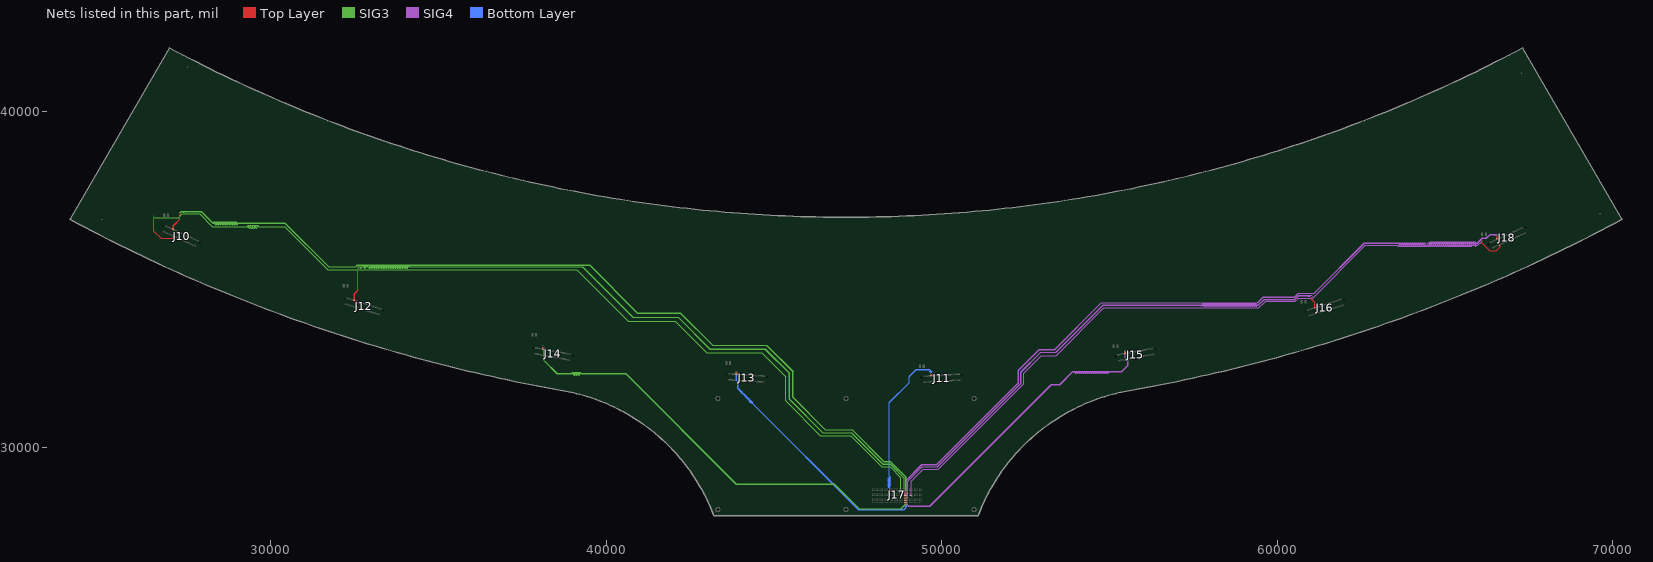
[diagram p0: the nets of this part, all layers, seen from the top]
# Altium PCB MISC86329.PcbDoc (part 4 of 11)
Units mil, origin at the board's own origin, x right, y up, seen from the top; angles counter-clockwise.
Board outline 46247.15 x 13937.21 mil, 6 copper layers (Top Layer, GND2, SIG3, SIG4, POWER5, Bottom Layer); 17 components, 210 nets, 908 pads, 1109 vias.

## Via types
v1: diameter 24, hole 12, Top Layer to Bottom Layer, 684 vias
v2: diameter 18, hole 9, Top Layer to Bottom Layer, 425 vias

## Nets (pads, with @x,y where several pads share a name; then routed paths per layer and width w, separated by ;. In a path a pad name is that pad's centre, name@x,y a point inside that pad or via, vN(x,y) a via of type N, cw(c..) or ccw(c..) an arc to the next point about the centre after c; other vN are vias at no path point) (continued)
DATAIN1P_CH7: J17.E7 J18.15 | length 23896.2
  Top Layer w5: J17.E7@49087.89,28568.8 v2(49111.69,28545) ; 66093,36150.5 66093,36104 66333,35864 66527,35864 66644,35981 66644,36016.48 J18.15@66618.61,36041.87
  SIG4 w5: v2(49111.69,28545) 49091.69,28565 49091.69,28998 49444.69,29351 49892.14,29351 52448,31906.86 52448,32213.86 52969.14,32735 53408.14,32735 54832.14,34159 59452.14,34159 59651.14,34358 60542.14,34358 60640.14,34456 61055.14,34456 62623.14,36024 63571.86,36024 63594.86,36001 63616.14,36001 63631.5,36016.36 63631.5,36049.43 63636.07,36054 63646.93,36054 63651.5,36049.43 63651.5,36004.43 63661.93,35994 63681.07,35994 63691.5,36004.43 63691.5,36049.43 63696.07,36054 63706.93,36054 63711.5,36049.43 63711.5,36004.43 63721.93,35994 63741.07,35994 63751.5,36004.43 63751.5,36049.43 63756.07,36054 63766.93,36054 63771.5,36049.43 63771.5,36004.43 63781.93,35994 63801.07,35994 63811.5,36004.43 63811.5,36049.43 63816.07,36054 63826.93,36054 63831.5,36049.43 63831.5,36004.43 63841.93,35994 63861.07,35994 63871.5,36004.43 63871.5,36049.43 63876.07,36054 63886.93,36054 63891.5,36049.43 63891.5,36004.43 63901.93,35994 63921.07,35994 63931.5,36004.43 63931.5,36049.43 63936.07,36054 63946.93,36054 63951.5,36049.43 63951.5,36004.43 63961.93,35994 63981.07,35994 63991.5,36004.43 63991.5,36049.43 63996.07,36054 64006.93,36054 64011.5,36049.43 64011.5,36004.43 64021.93,35994 64041.07,35994 64051.5,36004.43 64051.5,36049.43 64056.07,36054 64066.93,36054 64071.5,36049.43 64071.5,36004.43 64081.93,35994 64101.07,35994 64111.5,36004.43 64111.5,36049.43 64116.07,36054 64126.93,36054 64131.5,36049.43 64131.5,36004.43 64141.93,35994 64161.07,35994 64171.5,36004.43 64171.5,36049.43 64176.07,36054 64186.93,36054 64191.5,36049.43 64191.5,36004.43 64201.93,35994 64221.07,35994 64231.5,36004.43 64231.5,36049.43 64236.07,36054 64246.93,36054 64251.5,36049.43 64251.5,36004.43 64261.93,35994 64281.07,35994 64291.5,36004.43 64291.5,36049.43 64296.07,36054 64306.93,36054 64311.5,36049.43 64311.5,36004.43 64321.93,35994 64341.07,35994 64351.5,36004.43 64351.5,36049.43 64356.07,36054 64366.93,36054 64371.5,36049.43 64371.5,36004.43 64381.93,35994 64401.07,35994 64411.5,36004.43 64411.5,36019.43 64416.07,36024 64426.93,36024 64431.5,36019.43 64431.5,36004.43 64441.93,35994 64461.07,35994 64471.5,36004.43 64471.5,36019.43 64476.07,36024 64486.93,36024 64491.5,36019.43 64491.5,36004.43 64501.93,35994 64521.07,35994 64531.5,36004.43 64531.5,36049.43 64536.07,36054 64546.93,36054 64551.5,36049.43 64551.5,36004.43 64561.93,35994 64581.07,35994 64591.5,36004.43 64591.5,36019.43 64596.07,36024 64606.93,36024 64611.5,36019.43 64611.5,36004.43 64621.93,35994 64641.07,35994 64651.5,36004.43 64651.5,36019.43 64656.07,36024 64666.93,36024 64671.5,36019.43 64671.5,36004.43 64681.93,35994 64701.07,35994 64711.5,36004.43 64711.5,36019.43 64716.07,36024 64726.93,36024 64731.5,36019.43 64731.5,36004.43 64741.93,35994 64761.07,35994 64771.5,36004.43 64771.5,36019.43 64776.07,36024 64786.93,36024 64791.5,36019.43 64791.5,36004.43 64801.93,35994 64821.07,35994 64831.5,36004.43 64831.5,36019.43 64836.07,36024 64846.93,36024 64851.5,36019.43 64851.5,36004.43 64861.93,35994 64881.07,35994 64891.5,36004.43 64891.5,36019.43 64896.07,36024 64906.93,36024 64911.5,36019.43 64911.5,36004.43 64921.93,35994 64941.07,35994 64951.5,36004.43 64951.5,36019.43 64956.07,36024 64966.93,36024 64971.5,36019.43 64971.5,36004.43 64981.93,35994 65001.07,35994 65011.5,36004.43 65011.5,36019.43 65016.07,36024 65026.93,36024 65031.5,36019.43 65031.5,36004.43 65041.93,35994 65061.07,35994 65071.5,36004.43 65071.5,36019.43 65076.07,36024 65086.93,36024 65091.5,36019.43 65091.5,36004.43 65101.93,35994 65121.07,35994 65131.5,36004.43 65131.5,36019.43 65136.07,36024 65146.93,36024 65151.5,36019.43 65151.5,36004.43 65161.93,35994 65181.07,35994 65191.5,36004.43 65191.5,36019.43 65196.07,36024 65206.93,36024 65211.5,36019.43 65211.5,36004.43 65221.93,35994 65241.07,35994 65251.5,36004.43 65251.5,36019.43 65256.07,36024 65266.93,36024 65271.5,36019.43 65271.5,36004.43 65281.93,35994 65301.07,35994 65311.5,36004.43 65311.5,36019.43 65316.07,36024 65326.93,36024 65331.5,36019.43 65331.5,36004.43 65341.93,35994 65361.07,35994 65371.5,36004.43 65371.5,36019.43 65376.07,36024 65386.93,36024 65391.5,36019.43 65391.5,36004.43 65401.93,35994 65421.07,35994 65431.5,36004.43 65431.5,36019.43 65436.07,36024 65446.93,36024 65451.5,36019.43 65451.5,36004.43 65461.93,35994 65481.07,35994 65491.5,36004.43 65491.5,36019.43 65496.07,36024 65506.93,36024 65511.5,36019.43 65511.5,36004.43 65521.93,35994 65541.07,35994 65551.5,36004.43 65551.5,36019.43 65556.07,36024 65566.93,36024 65571.5,36019.43 65571.5,36004.43 65581.93,35994 65601.07,35994 65611.5,36004.43 65611.5,36019.43 65616.07,36024 65626.93,36024 65631.5,36019.43 65631.5,36004.43 65641.93,35994 65661.07,35994 65671.5,36004.43 65671.5,36019.43 65676.07,36024 65686.93,36024 65691.5,36019.43 65691.5,36004.43 65701.93,35994 65721.07,35994 65731.5,36004.43 65731.5,36019.43 65736.07,36024 65746.93,36024 65751.5,36019.43 65751.5,36004.43 65761.93,35994 65781.07,35994 65791.5,36004.43 65791.5,36019.43 65796.07,36024 65893,36024 65898,36019 65898,36007.06 65903,36002.06 65913,36002.06 65918,36007.06 65918,36019 65923,36024 65980,36024 66093,36137 66093,36143 ; 66093,36146 66093,36143 ; v2@66100,36157 66093,36150 66093,36143
  other v2: 66099.5,36157
DATAIN2N_CH0: J10.18 J17.G11 | length 27866.7
  Top Layer w5: J10.18@27107.16,36497.31 27107.16,36524.91 27120,36537.75 27120,36615 27304,36799 27304,36956.5 v2(27310.5,36963) ; J17.G11@48887.89,28668.8 v2(48911.69,28692.61)
  SIG3 w5: v2(27310.5,36963) 27304,36969.5 27304,36986 27347,37029 27388,37029 27403,37029 27408,37024 27408,37014.52 27413,37009.52 27423,37009.52 27428,37014.52 27428,37024 27433,37029 27935.86,37029 28280.86,36684 28313.82,36684 28325.5,36695.68 28325.5,36718.18 28331.32,36724 28344.68,36724 28350.5,36718.18 28350.5,36655.68 28362.18,36644 28383.82,36644 28395.5,36655.68 28395.5,36718.18 28401.32,36724 28414.68,36724 28420.5,36718.18 28420.5,36655.68 28432.18,36644 28453.82,36644 28465.5,36655.68 28465.5,36718.18 28471.32,36724 28484.68,36724 28490.5,36718.18 28490.5,36655.68 28502.18,36644 28523.82,36644 28535.5,36655.68 28535.5,36718.18 28541.32,36724 28554.68,36724 28560.5,36718.18 28560.5,36655.68 28572.18,36644 28593.82,36644 28605.5,36655.68 28605.5,36718.18 28611.32,36724 28624.68,36724 28630.5,36718.18 28630.5,36655.68 28642.18,36644 28663.82,36644 28675.5,36655.68 28675.5,36718.18 28681.32,36724 28694.68,36724 28700.5,36718.18 28700.5,36655.68 28712.18,36644 28733.82,36644 28745.5,36655.68 28745.5,36718.18 28751.32,36724 28764.68,36724 28770.5,36718.18 28770.5,36655.68 28782.18,36644 28803.82,36644 28815.5,36655.68 28815.5,36718.18 28821.32,36724 28834.68,36724 28840.5,36718.18 28840.5,36655.68 28852.18,36644 28873.82,36644 28885.5,36655.68 28885.5,36718.18 28891.32,36724 28904.68,36724 28910.5,36718.18 28910.5,36655.68 28922.18,36644 28943.82,36644 28955.5,36655.68 28955.5,36718.18 28961.32,36724 28974.68,36724 28980.5,36718.18 28980.5,36655.68 28992.18,36644 29013.82,36644 29025.5,36655.68 29025.5,36678.18 29031.32,36684 30428.86,36684 31731.86,35381 32545.14,35381 32596.14,35432 39506.86,35432 40930.86,34008 42208.86,34008 43173.86,33043 44780,33043 45560,32263 45560,31492.86 46528.86,30524 47328.86,30524 48274.86,29578 48465,29578 48931.69,29111.31 48931.69,28712.61 v2(48911.69,28692.61)
DATAIN2N_CH1: J12.18 J17.F11 | length 23094.8
  Top Layer w5: J12.18@32516.49,34376.54 32516.49,34403 32511,34408.49 32511,34584 32607,34680 32607,35344.5 v2(32613.5,35351) ; J17.F11@48887.89,28618.8 v2(48911.69,28642.61)
  SIG3 w5: v2(32613.5,35351) 32607,35357.5 32607,35366.86 32622.14,35382 32643,35382 32655.5,35382 32674.25,35382 32680.5,35375.75 32680.5,35349.42 32686.75,35343.17 32699.25,35343.17 32705.5,35349.42 32705.5,35375.75 32711.75,35382 32760.82,35382 32772.5,35393.68 32772.5,35406.18 32778.32,35412 32791.68,35412 32797.5,35406.18 32797.5,35354.13 32809.18,35342.46 32830.82,35342.46 32842.5,35354.13 32842.5,35406.18 32848.32,35412 32861.68,35412 32867.5,35406.18 32867.5,35393.68 32879.18,35382 32913,35382 32927.18,35382 32933,35376.18 32933,35354.13 32944.68,35342.46 32966.32,35342.46 32978,35354.13 32978,35406.18 32983.82,35412 32997.18,35412 33003,35406.18 33003,35354.13 33014.68,35342.46 33036.32,35342.46 33048,35354.13 33048,35406.18 33053.82,35412 33067.18,35412 33073,35406.18 33073,35354.13 33084.68,35342.46 33106.32,35342.46 33118,35354.13 33118,35406.18 33123.82,35412 33137.18,35412 33143,35406.18 33143,35354.13 33154.68,35342.46 33176.32,35342.46 33188,35354.13 33188,35406.18 33193.82,35412 33207.18,35412 33213,35406.18 33213,35354.13 33224.68,35342.46 33246.32,35342.46 33258,35354.13 33258,35406.18 33263.82,35412 33277.18,35412 33283,35406.18 33283,35354.13 33294.68,35342.46 33316.32,35342.46 33328,35354.13 33328,35406.18 33333.82,35412 33347.18,35412 33353,35406.18 33353,35354.13 33364.68,35342.46 33386.32,35342.46 33398,35354.13 33398,35406.18 33403.82,35412 33417.18,35412 33423,35406.18 33423,35354.13 33434.68,35342.46 33456.32,35342.46 33468,35354.13 33468,35406.18 33473.82,35412 33487.18,35412 33493,35406.18 33493,35354.13 33504.68,35342.46 33526.32,35342.46 33538,35354.13 33538,35406.18 33543.82,35412 33557.18,35412 33563,35406.18 33563,35354.13 33574.68,35342.46 33596.32,35342.46 33608,35354.13 33608,35406.18 33613.82,35412 33627.18,35412 33633,35406.18 33633,35354.13 33644.68,35342.46 33666.32,35342.46 33678,35354.13 33678,35406.18 33683.82,35412 33697.18,35412 33703,35406.18 33703,35354.13 33714.68,35342.46 33736.32,35342.46 33748,35354.13 33748,35406.18 33753.82,35412 33767.18,35412 33773,35406.18 33773,35354.13 33784.68,35342.46 33806.32,35342.46 33818,35354.13 33818,35406.18 33823.82,35412 33837.18,35412 33843,35406.18 33843,35354.13 33854.68,35342.46 33876.32,35342.46 33888,35354.13 33888,35406.18 33893.82,35412 33907.18,35412 33913,35406.18 33913,35354.13 33924.68,35342.46 33946.32,35342.46 33958,35354.13 33958,35406.18 33963.82,35412 33977.18,35412 33983,35406.18 33983,35354.13 33994.68,35342.46 34016.32,35342.46 34028,35354.13 34028,35406.18 34033.82,35412 34047.18,35412 34053,35406.18 34053,35354.13 34064.68,35342.46 34086.32,35342.46 34098,35354.13 34098,35406.18 34103.82,35412 34117.18,35412 34123,35406.18 34123,35393.68 34134.68,35382 39295.86,35382 40801.86,33876 42143.86,33876 43088.86,32931 44733,32931 45456,32208 45456,31434.86 46452.86,30438 47310.86,30438 48246.86,29502 48464,29502 48881,29085 48881,28676 48904.96,28652.04 48911.69,28645.31 v2(48911.69,28642.61)
DATAIN2N_CH2: J14.18 J17.B11 | length 13802
  Top Layer w5: v2(38142.5,33020) 38136,33013.5 38136,32958 38143.96,32950.04 J14.18@38143.96,32930.8 ; J17.B11@48887.89,28418.8 v2(48911.69,28395)
  SIG3 w5: v2@38142,33018 38136,33012 38136,32962.14 38146,32952.14 38146,32926.75 38152.25,32920.5 38157.54,32920.5 38163.79,32914.25 38163.79,32901.75 38157.54,32895.5 38152.25,32895.5 38146,32889.25 38146,32606 38541,32211 38988.68,32211 38994.5,32216.82 38994.5,32239.32 39006.18,32251 39027.82,32251 39039.5,32239.32 39039.5,32176.82 39045.32,32171 39058.68,32171 39064.5,32176.82 39064.5,32239.32 39076.18,32251 39097.82,32251 39109.5,32239.32 39109.5,32176.82 39115.32,32171 39128.68,32171 39134.5,32176.82 39134.5,32239.32 39146.18,32251 39167.82,32251 39179.5,32239.32 39179.5,32176.82 39185.32,32171 39198.68,32171 39204.5,32176.82 39204.5,32239.32 39216.18,32251 39237.82,32251 39249.5,32239.32 39249.5,32216.82 39255.32,32211 40584,32211 43873,28922 46805,28922 47547,28180 48783.69,28180 48931.69,28328 48931.69,28375 v2(48911.69,28395)
DATAIN2N_CH3: J13.18 J17.A11 | length 7737.2
  Top Layer w5: v2(43901.45,32250) 43894.95,32243.5 43894.95,32220.72 43905.67,32210 J13.18@43905.67,32181.66 ; J17.A11@48887.89,28368.8 v2(48911.69,28345)
  Bottom Layer w5: v2@43901,32247 43895,32241 43895,32204.75 43901.25,32198.5 43907.59,32198.5 43913.84,32192.25 43913.84,32179.75 43907.59,32173.5 43901.25,32173.5 43895,32167.25 43895,32001 43931,31965 43931,31754 43943.45,31741.55 43948.15,31741.55 43953.45,31746.85 43966.44,31746.85 43978.2,31735.08 43978.2,31722.1 43972.9,31716.8 43972.9,31712.1 43978.81,31706.19 43983.51,31706.19 43988.81,31711.49 44001.79,31711.49 44013.56,31699.73 44013.56,31686.74 44008.26,31681.44 44008.26,31676.74 44014.17,31670.83 44018.86,31670.83 44024.17,31676.14 44037.15,31676.14 44048.91,31664.37 44048.91,31651.39 44043.61,31646.09 44043.61,31641.39 44049.52,31635.48 44054.22,31635.48 44059.52,31640.78 44072.5,31640.78 44084.27,31629.01 44084.27,31616.03 44078.97,31610.73 44078.97,31606.03 44084.88,31600.12 44089.57,31600.12 44094.88,31605.43 44107.86,31605.43 44119.62,31593.66 44119.62,31580.68 44114.32,31575.38 44114.32,31570.68 44120.23,31564.77 44124.93,31564.77 44130.23,31570.07 44143.21,31570.07 44154.98,31558.3 44154.98,31545.32 44149.68,31540.02 44149.68,31535.32 44155.59,31529.41 44160.28,31529.41 44165.59,31534.72 44178.57,31534.72 44190.34,31522.95 44190.34,31509.97 44185.03,31504.66 44185.03,31499.97 44190.94,31494.06 44195.64,31494.06 44200.94,31499.36 44213.92,31499.36 44225.69,31487.59 44225.69,31474.61 44220.39,31469.31 44220.39,31464.61 44226.3,31458.7 44230.99,31458.7 44236.3,31464.01 44249.28,31464.01 44261.05,31452.24 44261.05,31439.26 44255.74,31433.95 44255.74,31429.26 44261.65,31423.35 44266.35,31423.35 44271.65,31428.65 44284.63,31428.65 44296.4,31416.88 44296.4,31403.9 44276.96,31384.46 44276.96,31379.76 44282.87,31373.85 44287.56,31373.85 44307.01,31393.29 44319.99,31393.29 44331.76,31381.53 44331.76,31368.55 44312.31,31349.1 44312.31,31344.4 44318.22,31338.49 44322.92,31338.49 44342.36,31357.94 44355.34,31357.94 44367.11,31346.17 44367.11,31333.19 44361.81,31327.89 44361.81,31323.19 47525,28160 48880,28160 48931.69,28211.69 48931.69,28228.18 48928.37,28231.5 48920.87,28231.5 48911.69,28240.68 48911.69,28257.32 48920.87,28266.5 48948.37,28266.5 48951.69,28269.82 48951.69,28278.18 48948.37,28281.5 48940.87,28281.5 48931.69,28290.68 48931.69,28325 v2(48911.69,28345)
DATAIN2N_CH4: J11.18 J17.H20 | length 5091.6
  Top Layer w5: v2(48414.09,28742.61) J17.H20@48437.89,28718.8 ; 49705.01,32196.5 49705.01,32175.72 49715.73,32165 J11.18@49715.73,32140.28
  Bottom Layer w5: v2(48414.09,28742.61) 48434.09,28762.61 48434.09,28813.93 48431.02,28817 48413.02,28817 48404.09,28825.93 48404.09,28848.07 48413.02,28857 48461.02,28857 48464.09,28860.07 48464.09,28873.93 48461.02,28877 48413.02,28877 48404.09,28885.93 48404.09,28908.07 48413.02,28917 48461.02,28917 48464.09,28920.07 48464.09,28933.93 48461.02,28937 48413.02,28937 48404.09,28945.93 48404.09,28968.07 48413.02,28977 48461.02,28977 48464.09,28980.07 48464.09,28993.93 48461.02,28997 48413.02,28997 48404.09,29005.93 48404.09,29028.07 48413.02,29037 48461.02,29037 48464.09,29040.07 48464.09,29053.93 48461.02,29057 48413.02,29057 48404.09,29065.93 48404.09,29088.07 48413.02,29097 48461.02,29097 48464.09,29100.07 48464.09,29113.93 48461.02,29117 48434.09,29143.91 48434.09,31343.09 49028,31937 49028,32120 49239,32331 49631.14,32331 49705,32257.14 49705,32210 v2@49713,32202
  other v2: 49711.51,32203
DATAIN2N_CH5: J15.18 J17.C11 | length 10126
  Top Layer w5: J17.C11@48887.89,28468.8 v2(48911.69,28445) ; 55474,32875.5 55474,32846.53 55487.53,32833 J15.18@55487.53,32807.27
  SIG4 w5: v2(48911.69,28445) 48933,28423.69 48933,28324.86 49000.86,28257 49653.14,28257 53274.14,31878 53526.14,31878 53908.14,32260 53967.43,32260 53972,32255.43 53972,32231.38 53982.43,32220.95 54001.57,32220.95 54012,32231.38 54012,32255.43 54016.57,32260 54027.43,32260 54032,32255.43 54032,32231.38 54042.43,32220.95 54061.57,32220.95 54072,32231.38 54072,32255.43 54076.57,32260 54087.43,32260 54092,32255.43 54092,32231.38 54102.43,32220.95 54121.57,32220.95 54132,32231.38 54132,32255.43 54136.57,32260 54147.43,32260 54152,32255.43 54152,32231.38 54162.43,32220.95 54181.57,32220.95 54192,32231.38 54192,32255.43 54196.57,32260 54207.43,32260 54212,32255.43 54212,32231.38 54222.43,32220.95 54241.57,32220.95 54252,32231.38 54252,32255.43 54256.57,32260 54267.43,32260 54272,32255.43 54272,32231.38 54282.43,32220.95 54301.57,32220.95 54312,32231.38 54312,32255.43 54316.57,32260 54327.43,32260 54332,32255.43 54332,32231.38 54342.43,32220.95 54361.57,32220.95 54372,32231.38 54372,32255.43 54376.57,32260 54387.43,32260 54392,32255.43 54392,32231.38 54402.43,32220.95 54421.57,32220.95 54432,32231.38 54432,32255.43 54436.57,32260 54447.43,32260 54452,32255.43 54452,32231.38 54462.43,32220.95 54481.57,32220.95 54492,32231.38 54492,32255.43 54496.57,32260 54507.43,32260 54512,32255.43 54512,32231.38 54522.43,32220.95 54541.57,32220.95 54552,32231.38 54552,32255.43 54556.57,32260 54567.43,32260 54572,32255.43 54572,32231.38 54582.43,32220.95 54601.57,32220.95 54612,32231.38 54612,32255.43 54616.57,32260 54627.43,32260 54632,32255.43 54632,32231.38 54642.43,32220.95 54661.57,32220.95 54672,32231.38 54672,32255.43 54676.57,32260 54687.43,32260 54692,32255.43 54692,32231.38 54702.43,32220.95 54721.57,32220.95 54732,32231.38 54732,32255.43 54736.57,32260 54747.43,32260 54752,32255.43 54752,32231.38 54762.43,32220.95 54781.57,32220.95 54792,32231.38 54792,32255.43 54796.57,32260 54807.43,32260 54812,32255.43 54812,32231.38 54822.43,32220.95 54841.57,32220.95 54852,32231.38 54852,32255.43 54856.57,32260 54867.43,32260 54872,32255.43 54872,32231.38 54882.43,32220.95 54901.57,32220.95 54912,32231.38 54912,32255.43 54916.57,32260 54927.43,32260 54932,32255.43 54932,32231.38 54942.43,32220.95 54961.57,32220.95 54972,32231.38 54972,32255.43 54976.57,32260 55371,32260 55561,32450 55561,32580.14 55474,32667.14 55474,32765 55474,32795 55474,32825 55474,32840 55474,32850 55474,32876 v2@55478,32880
  other v2: 55480.5,32882
DATAIN2N_CH6: J16.18 J17.D11 | length 18294.2
  Top Layer w5: J17.D11@48887.89,28518.8 v2(48911.69,28495) ; 61030,34491.5 61030,34416 61119,34327 61119,34188.72 J16.18@61135.02,34172.7
  SIG4 w5: v2(48911.69,28495) 48938.36,28495 48954.86,28511.5 48964.05,28511.5 48982,28529.45 48982,28994.14 49420.86,29433 49872,29433 52362,31923 52362,32254 52952,32844 53404,32844 54809,34249 57710,34249 57730,34229 57750.86,34229 57763,34241.14 57763,34268.57 57773.43,34279 57792.57,34279 57803,34268.57 57803,34223.57 57807.57,34219 57818.43,34219 57823,34223.57 57823,34268.57 57833.43,34279 57852.57,34279 57863,34268.57 57863,34223.57 57867.57,34219 57878.43,34219 57883,34223.57 57883,34268.57 57893.43,34279 57912.57,34279 57923,34268.57 57923,34223.57 57927.57,34219 57938.43,34219 57943,34223.57 57943,34268.57 57953.43,34279 57972.57,34279 57983,34268.57 57983,34223.57 57987.57,34219 57998.43,34219 58003,34223.57 58003,34268.57 58013.43,34279 58032.57,34279 58043,34268.57 58043,34223.57 58047.57,34219 58058.43,34219 58063,34223.57 58063,34268.57 58073.43,34279 58092.57,34279 58103,34268.57 58103,34223.57 58107.57,34219 58118.43,34219 58123,34223.57 58123,34268.57 58133.43,34279 58152.57,34279 58163,34268.57 58163,34223.57 58167.57,34219 58178.43,34219 58183,34223.57 58183,34268.57 58193.43,34279 58212.57,34279 58223,34268.57 58223,34223.57 58227.57,34219 58238.43,34219 58243,34223.57 58243,34268.57 58253.43,34279 58272.57,34279 58283,34268.57 58283,34223.57 58287.57,34219 58298.43,34219 58303,34223.57 58303,34268.57 58313.43,34279 58332.57,34279 58343,34268.57 58343,34223.57 58347.57,34219 58358.43,34219 58363,34223.57 58363,34268.57 58373.43,34279 58392.57,34279 58403,34268.57 58403,34223.57 58407.57,34219 58418.43,34219 58423,34223.57 58423,34268.57 58433.43,34279 58452.57,34279 58463,34268.57 58463,34223.57 58467.57,34219 58478.43,34219 58483,34223.57 58483,34268.57 58493.43,34279 58512.57,34279 58523,34268.57 58523,34223.57 58527.57,34219 58538.43,34219 58543,34223.57 58543,34268.57 58553.43,34279 58572.57,34279 58583,34268.57 58583,34223.57 58587.57,34219 58598.43,34219 58603,34223.57 58603,34268.57 58613.43,34279 58632.57,34279 58643,34268.57 58643,34223.57 58647.57,34219 58658.43,34219 58663,34223.57 58663,34268.57 58673.43,34279 58692.57,34279 58703,34268.57 58703,34223.57 58707.57,34219 58718.43,34219 58723,34223.57 58723,34268.57 58733.43,34279 58752.57,34279 58763,34268.57 58763,34223.57 58767.57,34219 58778.43,34219 58783,34223.57 58783,34268.57 58793.43,34279 58812.57,34279 58823,34268.57 58823,34223.57 58827.57,34219 58838.43,34219 58843,34223.57 58843,34268.57 58853.43,34279 58872.57,34279 58883,34268.57 58883,34223.57 58887.57,34219 58898.43,34219 58903,34223.57 58903,34268.57 58913.43,34279 58932.57,34279 58943,34268.57 58943,34223.57 58947.57,34219 58958.43,34219 58963,34223.57 58963,34268.57 58973.43,34279 58992.57,34279 59003,34268.57 59003,34223.57 59007.57,34219 59018.43,34219 59023,34223.57 59023,34268.57 59033.43,34279 59052.57,34279 59063,34268.57 59063,34223.57 59067.57,34219 59078.43,34219 59083,34223.57 59083,34268.57 59093.43,34279 59112.57,34279 59123,34268.57 59123,34223.57 59127.57,34219 59138.43,34219 59143,34223.57 59143,34268.57 59153.43,34279 59172.57,34279 59183,34268.57 59183,34223.57 59187.57,34219 59198.43,34219 59203,34223.57 59203,34268.57 59213.43,34279 59232.57,34279 59243,34268.57 59243,34223.57 59247.57,34219 59258.43,34219 59263,34223.57 59263,34268.57 59273.43,34279 59292.57,34279 59303,34268.57 59303,34223.57 59307.57,34219 59318.43,34219 59323,34223.57 59323,34268.57 59333.43,34279 59352.57,34279 59363,34268.57 59363,34223.57 59367.57,34219 59378.43,34219 59383,34223.57 59383,34238.57 59393.43,34249 59434.86,34249 59605.86,34420 60522,34420 60638,34536 61017.14,34536 61030,34523.14 61030,34509 61036,34503 v2@61036,34500
  other v2: 61036.5,34498
DATAIN2N_CH7: J17.E11 J18.18 | length 23893.9
  Top Layer w5: J17.E11@48887.89,28568.8 v2(48911.69,28545) ; 66555.34,36303.5 66555.34,36261.68 66564,36253.01 66564,36226.22 J18.18@66574.01,36216.2
  SIG4 w5: v2(48911.69,28545) 48931.69,28565 48931.69,29018.83 49412.86,29500 49854,29500 52286,31932 52286,32309.14 52905.86,32929 53366,32929 54755,34318 59409,34318 59581,34490 60516,34490 60631,34605 61104,34605 62597,36098 64392,36098 64411,36079 64477.86,36079 64496.86,36098 64538.43,36098 64543,36102.57 64543,36117.57 64553.43,36128 64572.57,36128 64583,36117.57 64583,36072.57 64587.57,36068 64598.43,36068 64603,36072.57 64603,36117.57 64613.43,36128 64632.57,36128 64643,36117.57 64643,36072.57 64647.57,36068 64658.43,36068 64663,36072.57 64663,36117.57 64673.43,36128 64692.57,36128 64703,36117.57 64703,36072.57 64707.57,36068 64718.43,36068 64723,36072.57 64723,36117.57 64733.43,36128 64752.57,36128 64763,36117.57 64763,36072.57 64767.57,36068 64778.43,36068 64783,36072.57 64783,36117.57 64793.43,36128 64812.57,36128 64823,36117.57 64823,36072.57 64827.57,36068 64838.43,36068 64843,36072.57 64843,36117.57 64853.43,36128 64872.57,36128 64883,36117.57 64883,36072.57 64887.57,36068 64898.43,36068 64903,36072.57 64903,36117.57 64913.43,36128 64932.57,36128 64943,36117.57 64943,36072.57 64947.57,36068 64958.43,36068 64963,36072.57 64963,36117.57 64973.43,36128 64992.57,36128 65003,36117.57 65003,36072.57 65007.57,36068 65018.43,36068 65023,36072.57 65023,36117.57 65033.43,36128 65052.57,36128 65063,36117.57 65063,36072.57 65067.57,36068 65078.43,36068 65083,36072.57 65083,36117.57 65093.43,36128 65112.57,36128 65123,36117.57 65123,36072.57 65127.57,36068 65138.43,36068 65143,36072.57 65143,36117.57 65153.43,36128 65172.57,36128 65183,36117.57 65183,36072.57 65187.57,36068 65198.43,36068 65203,36072.57 65203,36117.57 65213.43,36128 65232.57,36128 65243,36117.57 65243,36072.57 65247.57,36068 65258.43,36068 65263,36072.57 65263,36117.57 65273.43,36128 65292.57,36128 65303,36117.57 65303,36072.57 65307.57,36068 65318.43,36068 65323,36072.57 65323,36117.57 65333.43,36128 65352.57,36128 65363,36117.57 65363,36072.57 65367.57,36068 65378.43,36068 65383,36072.57 65383,36117.57 65393.43,36128 65412.57,36128 65423,36117.57 65423,36072.57 65427.57,36068 65438.43,36068 65443,36072.57 65443,36117.57 65453.43,36128 65472.57,36128 65483,36117.57 65483,36072.57 65487.57,36068 65498.43,36068 65503,36072.57 65503,36117.57 65513.43,36128 65532.57,36128 65543,36117.57 65543,36072.57 65547.57,36068 65558.43,36068 65563,36072.57 65563,36117.57 65573.43,36128 65592.57,36128 65603,36117.57 65603,36072.57 65607.57,36068 65618.43,36068 65623,36072.57 65623,36117.57 65633.43,36128 65652.57,36128 65663,36117.57 65663,36072.57 65667.57,36068 65678.43,36068 65683,36072.57 65683,36117.57 65693.43,36128 65712.57,36128 65723,36117.57 65723,36072.57 65727.57,36068 65738.43,36068 65743,36072.57 65743,36117.57 65753.43,36128 65772.57,36128 65783,36117.57 65783,36072.57 65787.57,36068 65798.43,36068 65803,36072.57 65803,36117.57 65813.43,36128 65832.57,36128 65843,36117.57 65843,36072.57 65847.57,36068 65858.43,36068 65863,36072.57 65863,36117.57 65873.43,36128 65892.57,36128 65903,36117.57 65903,36072.57 65907.57,36068 65918.43,36068 65923,36072.57 65923,36087.57 65933.43,36098 65964,36098 66114,36248 66233,36248 66343,36358 66533.14,36358 66556,36335.14 66556,36318 v2@66562,36312
  other v2: 66561.84,36310
DATAIN2P_CH0: J10.16 J17.G10 | length 27867.3
  Top Layer w5: J10.16@27078.52,36510.41 27110,36541.89 27110,36619.14 27294,36803.14 27294,36956.5 v2(27287.5,36963) ; J17.G10@48937.89,28668.8 v2(48961.69,28692.61)
  SIG3 w5: v2(27287.5,36963) 27294,36969.5 27294,36990.14 27342.86,37039 27388,37039 27403,37039 27940,37039 28285,36694 28309.68,36694 28315.5,36699.82 28315.5,36722.32 28327.18,36734 28348.82,36734 28360.5,36722.32 28360.5,36659.82 28366.32,36654 28379.68,36654 28385.5,36659.82 28385.5,36722.32 28397.18,36734 28418.82,36734 28430.5,36722.32 28430.5,36659.82 28436.32,36654 28449.68,36654 28455.5,36659.82 28455.5,36722.32 28467.18,36734 28488.82,36734 28500.5,36722.32 28500.5,36659.82 28506.32,36654 28519.68,36654 28525.5,36659.82 28525.5,36722.32 28537.18,36734 28558.82,36734 28570.5,36722.32 28570.5,36659.82 28576.32,36654 28589.68,36654 28595.5,36659.82 28595.5,36722.32 28607.18,36734 28628.82,36734 28640.5,36722.32 28640.5,36659.82 28646.32,36654 28659.68,36654 28665.5,36659.82 28665.5,36722.32 28677.18,36734 28698.82,36734 28710.5,36722.32 28710.5,36659.82 28716.32,36654 28729.68,36654 28735.5,36659.82 28735.5,36722.32 28747.18,36734 28768.82,36734 28780.5,36722.32 28780.5,36659.82 28786.32,36654 28799.68,36654 28805.5,36659.82 28805.5,36722.32 28817.18,36734 28838.82,36734 28850.5,36722.32 28850.5,36659.82 28856.32,36654 28869.68,36654 28875.5,36659.82 28875.5,36722.32 28887.18,36734 28908.82,36734 28920.5,36722.32 28920.5,36659.82 28926.32,36654 28939.68,36654 28945.5,36659.82 28945.5,36722.32 28957.18,36734 28978.82,36734 28990.5,36722.32 28990.5,36659.82 28996.32,36654 29009.68,36654 29015.5,36659.82 29015.5,36682.32 29027.18,36694 30433,36694 31736,35391 32541,35391 32592,35442 39511,35442 40935,34018 42213,34018 43178,33053 44784.14,33053 45570,32267.14 45570,31497 46533,30534 47333,30534 48279,29588 48469.14,29588 48941.69,29115.45 48941.69,28712.61 v2(48961.69,28692.61)
DATAIN2P_CH1: J12.16 J17.F10 | length 23095.2
  Top Layer w5: J12.16@32486.47,34386.04 32486.47,34396.47 32501,34411 32501,34588.14 32597,34684.14 32597,35344.5 v2(32590.5,35351) ; J17.F10@48937.89,28618.8 v2(48961.69,28642.61)
  SIG3 w5: v2(32590.5,35351) 32597,35357.5 32597,35371 32618,35392 32643,35392 32655.5,35392 32674.25,35392 32711.75,35392 32756.68,35392 32762.5,35397.82 32762.5,35410.32 32774.18,35422 32795.82,35422 32807.5,35410.32 32807.5,35358.28 32813.32,35352.46 32826.68,35352.46 32832.5,35358.28 32832.5,35410.32 32844.18,35422 32865.82,35422 32877.5,35410.32 32877.5,35397.82 32883.32,35392 32913,35392 32931.32,35392 32943,35380.32 32943,35358.28 32948.82,35352.46 32962.18,35352.46 32968,35358.28 32968,35410.32 32979.68,35422 33001.32,35422 33013,35410.32 33013,35358.28 33018.82,35352.46 33032.18,35352.46 33038,35358.28 33038,35410.32 33049.68,35422 33071.32,35422 33083,35410.32 33083,35358.28 33088.82,35352.46 33102.18,35352.46 33108,35358.28 33108,35410.32 33119.68,35422 33141.32,35422 33153,35410.32 33153,35358.28 33158.82,35352.46 33172.18,35352.46 33178,35358.28 33178,35410.32 33189.68,35422 33211.32,35422 33223,35410.32 33223,35358.28 33228.82,35352.46 33242.18,35352.46 33248,35358.28 33248,35410.32 33259.68,35422 33281.32,35422 33293,35410.32 33293,35358.28 33298.82,35352.46 33312.18,35352.46 33318,35358.28 33318,35410.32 33329.68,35422 33351.32,35422 33363,35410.32 33363,35358.28 33368.82,35352.46 33382.18,35352.46 33388,35358.28 33388,35410.32 33399.68,35422 33421.32,35422 33433,35410.32 33433,35358.28 33438.82,35352.46 33452.18,35352.46 33458,35358.28 33458,35410.32 33469.68,35422 33491.32,35422 33503,35410.32 33503,35358.28 33508.82,35352.46 33522.18,35352.46 33528,35358.28 33528,35410.32 33539.68,35422 33561.32,35422 33573,35410.32 33573,35358.28 33578.82,35352.46 33592.18,35352.46 33598,35358.28 33598,35410.32 33609.68,35422 33631.32,35422 33643,35410.32 33643,35358.28 33648.82,35352.46 33662.18,35352.46 33668,35358.28 33668,35410.32 33679.68,35422 33701.32,35422 33713,35410.32 33713,35358.28 33718.82,35352.46 33732.18,35352.46 33738,35358.28 33738,35410.32 33749.68,35422 33771.32,35422 33783,35410.32 33783,35358.28 33788.82,35352.46 33802.18,35352.46 33808,35358.28 33808,35410.32 33819.68,35422 33841.32,35422 33853,35410.32 33853,35358.28 33858.82,35352.46 33872.18,35352.46 33878,35358.28 33878,35410.32 33889.68,35422 33911.32,35422 33923,35410.32 33923,35358.28 33928.82,35352.46 33942.18,35352.46 33948,35358.28 33948,35410.32 33959.68,35422 33981.32,35422 33993,35410.32 33993,35358.28 33998.82,35352.46 34012.18,35352.46 34018,35358.28 34018,35410.32 34029.68,35422 34051.32,35422 34063,35410.32 34063,35358.28 34068.82,35352.46 34082.18,35352.46 34088,35358.28 34088,35410.32 34099.68,35422 34121.32,35422 34133,35410.32 34133,35397.82 34138.82,35392 39300,35392 40806,33886 42148,33886 43093,32941 44737.14,32941 45466,32212.14 45466,31439 46457,30448 47315,30448 48251,29512 48468.14,29512 48891,29089.14 48891,28680.14 48912.04,28659.11 48918.53,28659.11 48935.03,28642.61 v2(48961.69,28642.61)
DATAIN2P_CH2: J14.16 J17.B10 | length 13802.3
  Top Layer w5: J14.16@38113,32936.58 38113,32947 38126,32960 38126,33013.5 ; J17.B10@48937.89,28418.8 v2(48961.69,28395)
  SIG3 w5: v2@38120,33019 38126,33013 38126,32958 38136,32948 38136,32926.75 38136,32601.86 38536.86,32201 38992.82,32201 39004.5,32212.68 39004.5,32235.18 39010.32,32241 39023.68,32241 39029.5,32235.18 39029.5,32172.68 39041.18,32161 39062.82,32161 39074.5,32172.68 39074.5,32235.18 39080.32,32241 39093.68,32241 39099.5,32235.18 39099.5,32172.68 39111.18,32161 39132.82,32161 39144.5,32172.68 39144.5,32235.18 39150.32,32241 39163.68,32241 39169.5,32235.18 39169.5,32172.68 39181.18,32161 39202.82,32161 39214.5,32172.68 39214.5,32235.18 39220.32,32241 39233.68,32241 39239.5,32235.18 39239.5,32212.68 39251.18,32201 40579.86,32201 43868.86,28912 46800.86,28912 47542.86,28170 48787.83,28170 48941.69,28323.86 48941.69,28375 v2(48961.69,28395)
  other v2: 38119.5,33020
DATAIN2P_CH3: J13.16 J17.A10 | length 7738.2
  Top Layer w5: J13.16@43874.24,32183.62 43874.24,32210 43884.95,32220.72 43884.95,32243.5 ; J17.A10@48937.89,28368.8 v2(48961.69,28345)
  Bottom Layer w5: v2@43879,32249 43885,32243 43885,32204.75 43885,31996.86 43921,31960.86 43921,31749.86 43939.31,31731.55 43952.29,31731.55 43957.6,31736.85 43962.29,31736.85 43968.2,31730.94 43968.2,31726.24 43962.9,31720.94 43962.9,31707.96 43974.67,31696.19 43987.65,31696.19 43992.95,31701.49 43997.65,31701.49 44003.56,31695.58 44003.56,31690.89 43998.26,31685.58 43998.26,31672.6 44010.02,31660.83 44023,31660.83 44028.31,31666.14 44033,31666.14 44038.91,31660.23 44038.91,31655.53 44033.61,31650.23 44033.61,31637.25 44045.38,31625.48 44058.36,31625.48 44063.66,31630.78 44068.36,31630.78 44074.27,31624.87 44074.27,31620.18 44068.97,31614.87 44068.97,31601.89 44080.73,31590.12 44093.72,31590.12 44099.02,31595.43 44103.71,31595.43 44109.62,31589.52 44109.62,31584.82 44104.32,31579.52 44104.32,31566.54 44116.09,31554.77 44129.07,31554.77 44134.37,31560.07 44139.07,31560.07 44144.98,31554.16 44144.98,31549.47 44139.68,31544.16 44139.68,31531.18 44151.44,31519.41 44164.43,31519.41 44169.73,31524.72 44174.43,31524.72 44180.34,31518.81 44180.34,31514.11 44175.03,31508.81 44175.03,31495.83 44186.8,31484.06 44199.78,31484.06 44205.08,31489.36 44209.78,31489.36 44215.69,31483.45 44215.69,31478.75 44210.39,31473.45 44210.39,31460.47 44222.16,31448.7 44235.14,31448.7 44240.44,31454.01 44245.14,31454.01 44251.05,31448.1 44251.05,31443.4 44245.74,31438.1 44245.74,31425.11 44257.51,31413.35 44270.49,31413.35 44275.8,31418.65 44280.49,31418.65 44286.4,31412.74 44286.4,31408.04 44266.96,31388.6 44266.96,31375.62 44278.72,31363.85 44291.71,31363.85 44311.15,31383.29 44315.85,31383.29 44321.76,31377.39 44321.76,31372.69 44302.31,31353.24 44302.31,31340.26 44314.08,31328.49 44327.06,31328.49 44346.51,31347.94 44351.2,31347.94 44357.11,31342.03 44357.11,31337.33 44351.81,31332.03 44351.81,31319.05 47520.86,28150 48884.14,28150 48941.69,28207.55 48941.69,28232.32 48932.51,28241.5 48925.01,28241.5 48921.69,28244.82 48921.69,28253.18 48925.01,28256.5 48952.51,28256.5 48961.69,28265.68 48961.69,28282.32 48952.51,28291.5 48945.01,28291.5 48941.69,28294.82 48941.69,28325 v2(48961.69,28345)
  other v2: 43878.45,32250
DATAIN2P_CH4: J11.16 J17.H19 | length 5091.1
  Top Layer w5: v2(48464.09,28742.61) J17.H19@48487.89,28718.8 ; J11.16@49684.29,32138.39 49684.29,32164 49695.01,32174.72 49695.01,32196.5
  Bottom Layer w5: v2(48464.09,28742.61) 48444.09,28762.61 48444.09,28818.07 48435.16,28827 48417.16,28827 48414.09,28830.07 48414.09,28843.93 48417.16,28847 48465.16,28847 48474.09,28855.93 48474.09,28878.07 48465.16,28887 48417.16,28887 48414.09,28890.07 48414.09,28903.93 48417.16,28907 48465.16,28907 48474.09,28915.93 48474.09,28938.07 48465.16,28947 48417.16,28947 48414.09,28950.07 48414.09,28963.93 48417.16,28967 48465.16,28967 48474.09,28975.93 48474.09,28998.07 48465.16,29007 48417.16,29007 48414.09,29010.07 48414.09,29023.93 48417.16,29027 48465.16,29027 48474.09,29035.93 48474.09,29058.07 48465.16,29067 48417.16,29067 48414.09,29070.07 48414.09,29083.93 48417.16,29087 48465.16,29087 48474.09,29095.93 48474.09,29118.07 48465.16,29127 48444.09,29148.06 48444.09,31338.94 49038,31932.86 49038,32115.86 49243.14,32321 49627,32321 49660.75,32287.25 49660.75,32280.18 49651.79,32271.22 49651.79,32264.15 49658.86,32257.08 49665.94,32257.08 49674.89,32266.04 49681.96,32266.04 49695,32253 49695,32210 v2@49689,32204
  other v2: 49688.51,32203
DATAIN2P_CH5: J15.16 J17.C10 | length 10126
  Top Layer w5: J17.C10@48937.89,28468.8 v2(48961.69,28445) ; J15.16@55456.56,32801.57 55456.56,32828 55464,32835.44 55464,32875.5
  SIG4 w5: v2(48961.69,28445) 48943,28426.31 48943,28329 49005,28267 49649,28267 53270,31888 53522,31888 53904,32270 53971.57,32270 53982,32259.57 53982,32235.52 53986.57,32230.95 53997.43,32230.95 54002,32235.52 54002,32259.57 54012.43,32270 54031.57,32270 54042,32259.57 54042,32235.52 54046.57,32230.95 54057.43,32230.95 54062,32235.52 54062,32259.57 54072.43,32270 54091.57,32270 54102,32259.57 54102,32235.52 54106.57,32230.95 54117.43,32230.95 54122,32235.52 54122,32259.57 54132.43,32270 54151.57,32270 54162,32259.57 54162,32235.52 54166.57,32230.95 54177.43,32230.95 54182,32235.52 54182,32259.57 54192.43,32270 54211.57,32270 54222,32259.57 54222,32235.52 54226.57,32230.95 54237.43,32230.95 54242,32235.52 54242,32259.57 54252.43,32270 54271.57,32270 54282,32259.57 54282,32235.52 54286.57,32230.95 54297.43,32230.95 54302,32235.52 54302,32259.57 54312.43,32270 54331.57,32270 54342,32259.57 54342,32235.52 54346.57,32230.95 54357.43,32230.95 54362,32235.52 54362,32259.57 54372.43,32270 54391.57,32270 54402,32259.57 54402,32235.52 54406.57,32230.95 54417.43,32230.95 54422,32235.52 54422,32259.57 54432.43,32270 54451.57,32270 54462,32259.57 54462,32235.52 54466.57,32230.95 54477.43,32230.95 54482,32235.52 54482,32259.57 54492.43,32270 54511.57,32270 54522,32259.57 54522,32235.52 54526.57,32230.95 54537.43,32230.95 54542,32235.52 54542,32259.57 54552.43,32270 54571.57,32270 54582,32259.57 54582,32235.52 54586.57,32230.95 54597.43,32230.95 54602,32235.52 54602,32259.57 54612.43,32270 54631.57,32270 54642,32259.57 54642,32235.52 54646.57,32230.95 54657.43,32230.95 54662,32235.52 54662,32259.57 54672.43,32270 54691.57,32270 54702,32259.57 54702,32235.52 54706.57,32230.95 54717.43,32230.95 54722,32235.52 54722,32259.57 54732.43,32270 54751.57,32270 54762,32259.57 54762,32235.52 54766.57,32230.95 54777.43,32230.95 54782,32235.52 54782,32259.57 54792.43,32270 54811.57,32270 54822,32259.57 54822,32235.52 54826.57,32230.95 54837.43,32230.95 54842,32235.52 54842,32259.57 54852.43,32270 54871.57,32270 54882,32259.57 54882,32235.52 54886.57,32230.95 54897.43,32230.95 54902,32235.52 54902,32259.57 54912.43,32270 54931.57,32270 54942,32259.57 54942,32235.52 54946.57,32230.95 54957.43,32230.95 54962,32235.52 54962,32259.57 54972.43,32270 55366.86,32270 55551,32454.14 55551,32576 55464,32663 55464,32765 55464,32795 55459,32800 55448.15,32800 55443.15,32805 55443.15,32815 55448.15,32820 55459,32820 55464,32825 55464,32840 55464,32850 55464,32877 v2@55460,32881
  other v2: 55457.5,32882
DATAIN2P_CH6: J16.16 J17.D10 | length 18293.6
  Top Layer w5: J17.D10@48937.89,28518.8 v2(48961.69,28495) ; v2(61013.5,34498) 61020,34491.5 61020,34411.86 61109,34322.86 61109,34185 61104.97,34180.97 J16.16@61104.97,34163.26
  SIG4 w5: v2(48961.69,28495) 48992,28525.31 48992,28990 49425,29423 49876.14,29423 52372,31918.86 52372,32249.86 52956.14,32834 53408.14,32834 54813.14,34239 57705.86,34239 57725.86,34219 57755,34219 57773,34237 57773,34264.43 57777.57,34269 57788.43,34269 57793,34264.43 57793,34219.43 57803.43,34209 57822.57,34209 57833,34219.43 57833,34264.43 57837.57,34269 57848.43,34269 57853,34264.43 57853,34219.43 57863.43,34209 57882.57,34209 57893,34219.43 57893,34264.43 57897.57,34269 57908.43,34269 57913,34264.43 57913,34219.43 57923.43,34209 57942.57,34209 57953,34219.43 57953,34264.43 57957.57,34269 57968.43,34269 57973,34264.43 57973,34219.43 57983.43,34209 58002.57,34209 58013,34219.43 58013,34264.43 58017.57,34269 58028.43,34269 58033,34264.43 58033,34219.43 58043.43,34209 58062.57,34209 58073,34219.43 58073,34264.43 58077.57,34269 58088.43,34269 58093,34264.43 58093,34219.43 58103.43,34209 58122.57,34209 58133,34219.43 58133,34264.43 58137.57,34269 58148.43,34269 58153,34264.43 58153,34219.43 58163.43,34209 58182.57,34209 58193,34219.43 58193,34264.43 58197.57,34269 58208.43,34269 58213,34264.43 58213,34219.43 58223.43,34209 58242.57,34209 58253,34219.43 58253,34264.43 58257.57,34269 58268.43,34269 58273,34264.43 58273,34219.43 58283.43,34209 58302.57,34209 58313,34219.43 58313,34264.43 58317.57,34269 58328.43,34269 58333,34264.43 58333,34219.43 58343.43,34209 58362.57,34209 58373,34219.43 58373,34264.43 58377.57,34269 58388.43,34269 58393,34264.43 58393,34219.43 58403.43,34209 58422.57,34209 58433,34219.43 58433,34264.43 58437.57,34269 58448.43,34269 58453,34264.43 58453,34219.43 58463.43,34209 58482.57,34209 58493,34219.43 58493,34264.43 58497.57,34269 58508.43,34269 58513,34264.43 58513,34219.43 58523.43,34209 58542.57,34209 58553,34219.43 58553,34264.43 58557.57,34269 58568.43,34269 58573,34264.43 58573,34219.43 58583.43,34209 58602.57,34209 58613,34219.43 58613,34264.43 58617.57,34269 58628.43,34269 58633,34264.43 58633,34219.43 58643.43,34209 58662.57,34209 58673,34219.43 58673,34264.43 58677.57,34269 58688.43,34269 58693,34264.43 58693,34219.43 58703.43,34209 58722.57,34209 58733,34219.43 58733,34264.43 58737.57,34269 58748.43,34269 58753,34264.43 58753,34219.43 58763.43,34209 58782.57,34209 58793,34219.43 58793,34264.43 58797.57,34269 58808.43,34269 58813,34264.43 58813,34219.43 58823.43,34209 58842.57,34209 58853,34219.43 58853,34264.43 58857.57,34269 58868.43,34269 58873,34264.43 58873,34219.43 58883.43,34209 58902.57,34209 58913,34219.43 58913,34264.43 58917.57,34269 58928.43,34269 58933,34264.43 58933,34219.43 58943.43,34209 58962.57,34209 58973,34219.43 58973,34264.43 58977.57,34269 58988.43,34269 58993,34264.43 58993,34219.43 59003.43,34209 59022.57,34209 59033,34219.43 59033,34264.43 59037.57,34269 59048.43,34269 59053,34264.43 59053,34219.43 59063.43,34209 59082.57,34209 59093,34219.43 59093,34264.43 59097.57,34269 59108.43,34269 59113,34264.43 59113,34219.43 59123.43,34209 59142.57,34209 59153,34219.43 59153,34264.43 59157.57,34269 59168.43,34269 59173,34264.43 59173,34219.43 59183.43,34209 59202.57,34209 59213,34219.43 59213,34264.43 59217.57,34269 59228.43,34269 59233,34264.43 59233,34219.43 59243.43,34209 59262.57,34209 59273,34219.43 59273,34264.43 59277.57,34269 59288.43,34269 59293,34264.43 59293,34219.43 59303.43,34209 59322.57,34209 59333,34219.43 59333,34264.43 59337.57,34269 59348.43,34269 59353,34264.43 59353,34219.43 59363.43,34209 59382.57,34209 59393,34219.43 59393,34234.43 59397.57,34239 59439,34239 59610,34410 60526.14,34410 60642.14,34526 60898,34526 60903,34521 60903,34511.03 60908,34506.03 60918,34506.03 60923,34511.03 60923,34521 60928,34526 60938,34526 60943,34521 60943,34511.03 60948,34506.03 60958,34506.03 60963,34511.03 60963,34521 60968,34526 61013,34526 61020,34519 61020,34506 v2@61014,34500
DATAIN2P_CH7: J17.E10 J18.16 | length 23893.8
  Top Layer w5: J17.E10@48937.89,28568.8 v2(48961.69,28545) ; J18.16@66545.34,36203.18 66545.34,36303.5
  SIG4 w5: v2(48961.69,28545) 48941.69,28565 48941.69,29014.69 49417,29490 49858.14,29490 52296,31927.86 52296,32305 52910,32919 53370.14,32919 54759.14,34308 59413.14,34308 59585.14,34480 60520.14,34480 60635.14,34595 61108.14,34595 62601.14,36088 64387.86,36088 64406.86,36069 64482,36069 64501,36088 64542.57,36088 64553,36098.43 64553,36113.43 64557.57,36118 64568.43,36118 64573,36113.43 64573,36068.43 64583.43,36058 64602.57,36058 64613,36068.43 64613,36113.43 64617.57,36118 64628.43,36118 64633,36113.43 64633,36068.43 64643.43,36058 64662.57,36058 64673,36068.43 64673,36113.43 64677.57,36118 64688.43,36118 64693,36113.43 64693,36068.43 64703.43,36058 64722.57,36058 64733,36068.43 64733,36113.43 64737.57,36118 64748.43,36118 64753,36113.43 64753,36068.43 64763.43,36058 64782.57,36058 64793,36068.43 64793,36113.43 64797.57,36118 64808.43,36118 64813,36113.43 64813,36068.43 64823.43,36058 64842.57,36058 64853,36068.43 64853,36113.43 64857.57,36118 64868.43,36118 64873,36113.43 64873,36068.43 64883.43,36058 64902.57,36058 64913,36068.43 64913,36113.43 64917.57,36118 64928.43,36118 64933,36113.43 64933,36068.43 64943.43,36058 64962.57,36058 64973,36068.43 64973,36113.43 64977.57,36118 64988.43,36118 64993,36113.43 64993,36068.43 65003.43,36058 65022.57,36058 65033,36068.43 65033,36113.43 65037.57,36118 65048.43,36118 65053,36113.43 65053,36068.43 65063.43,36058 65082.57,36058 65093,36068.43 65093,36113.43 65097.57,36118 65108.43,36118 65113,36113.43 65113,36068.43 65123.43,36058 65142.57,36058 65153,36068.43 65153,36113.43 65157.57,36118 65168.43,36118 65173,36113.43 65173,36068.43 65183.43,36058 65202.57,36058 65213,36068.43 65213,36113.43 65217.57,36118 65228.43,36118 65233,36113.43 65233,36068.43 65243.43,36058 65262.57,36058 65273,36068.43 65273,36113.43 65277.57,36118 65288.43,36118 65293,36113.43 65293,36068.43 65303.43,36058 65322.57,36058 65333,36068.43 65333,36113.43 65337.57,36118 65348.43,36118 65353,36113.43 65353,36068.43 65363.43,36058 65382.57,36058 65393,36068.43 65393,36113.43 65397.57,36118 65408.43,36118 65413,36113.43 65413,36068.43 65423.43,36058 65442.57,36058 65453,36068.43 65453,36113.43 65457.57,36118 65468.43,36118 65473,36113.43 65473,36068.43 65483.43,36058 65502.57,36058 65513,36068.43 65513,36113.43 65517.57,36118 65528.43,36118 65533,36113.43 65533,36068.43 65543.43,36058 65562.57,36058 65573,36068.43 65573,36113.43 65577.57,36118 65588.43,36118 65593,36113.43 65593,36068.43 65603.43,36058 65622.57,36058 65633,36068.43 65633,36113.43 65637.57,36118 65648.43,36118 65653,36113.43 65653,36068.43 65663.43,36058 65682.57,36058 65693,36068.43 65693,36113.43 65697.57,36118 65708.43,36118 65713,36113.43 65713,36068.43 65723.43,36058 65742.57,36058 65753,36068.43 65753,36113.43 65757.57,36118 65768.43,36118 65773,36113.43 65773,36068.43 65783.43,36058 65802.57,36058 65813,36068.43 65813,36113.43 65817.57,36118 65828.43,36118 65833,36113.43 65833,36068.43 65843.43,36058 65862.57,36058 65873,36068.43 65873,36113.43 65877.57,36118 65888.43,36118 65893,36113.43 65893,36068.43 65903.43,36058 65922.57,36058 65933,36068.43 65933,36083.43 65937.57,36088 65968.14,36088 66118.14,36238 66237.14,36238 66347.14,36348 66471,36348 66476,36343 66476,36336.27 66481,36331.27 66491,36331.27 66496,36336.27 66496,36343 66501,36348 66529,36348 66546,36331 66546,36322 ; v2(66538.84,36310) v2@66539,36310.16 ; v2@66539,36309 v2@66539,36310.16 ; v2@66539,36310.5 v2@66539,36310.16 ; 66546,36320 66546,36322 ; v2@66539,36310.16 66545.34,36316.5 66545.34,36316.83 66546,36317.5 66546,36322
DATAIN3N_CH0: J10.23 J17.G14 | length 28227.3
  Top Layer w5: v2(26522.5,36894) 26529,36887.5 26529,36447.86 26742.86,36234 27070.14,36234 27100.78,36264.64 27100.78,36278.25 J10.23@27119.43,36296.9 ; J17.G14@48737.89,28668.8 v2(48761.69,28692.61)
  SIG3 w5: v2(26522.5,36894) 26529,36887.5 26529,36867.86 26544.86,36852 26580,36852 27261,36852 27369,36960 27886.86,36960 28267.86,36579 29315.82,36579 29327.5,36590.68 29327.5,36612.41 29333.32,36618.24 29346.68,36618.24 29352.5,36612.41 29352.5,36551.44 29364.18,36539.76 29385.82,36539.76 29397.5,36551.44 29397.5,36612.41 29403.32,36618.24 29416.68,36618.24 29422.5,36612.41 29422.5,36551.44 29434.18,36539.76 29455.82,36539.76 29467.5,36551.44 29467.5,36612.41 29473.32,36618.24 29486.68,36618.24 29492.5,36612.41 29492.5,36551.44 29504.18,36539.76 29525.82,36539.76 29537.5,36551.44 29537.5,36612.41 29543.32,36618.24 29556.68,36618.24 29562.5,36612.41 29562.5,36551.44 29574.18,36539.76 29595.82,36539.76 29607.5,36551.44 29607.5,36612.41 29613.32,36618.24 29626.68,36618.24 29632.5,36612.41 29632.5,36590.68 29644.18,36579 30428.86,36579 31708.86,35299 39131.86,35299 40667.86,33763 42058.86,33763 42994.86,32827 44634,32827 45352,32109 45352,31389.86 46387.86,30354 47283.86,30354 48214.86,29423 48463,29423 48781.69,29104.31 48781.69,28712.61 v2(48761.69,28692.61)